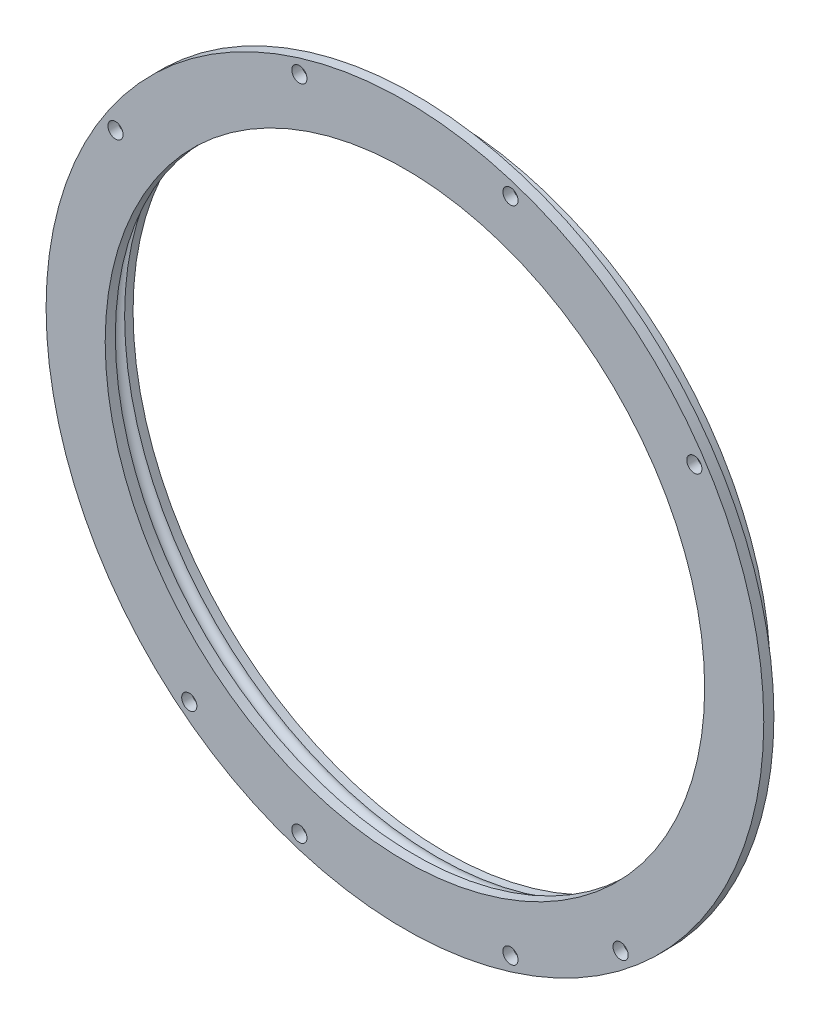
SolidWorks part; units mm, degrees
ref_plane "前视基准面" through (0, 0, 0) normal (0, 0, 1) x (1, 0, 0)
ref_plane "上视基准面" through (0, 0, 0) normal (0, 1, 0) x (1, 0, 0)
ref_plane "右视基准面" through (0, 0, 0) normal (1, 0, 0) x (0, 0, -1)
sketch "草图1" plane through (0, 0, 0) normal (0, 0, 1) x (1, 0, 0)
  circle A0 centre (0, 0) radius 425
  circle A1 centre (0, 0) radius 355
  circle A2 centre (0, 0) radius 409 construction
  dimension "D1" = 850
  dimension "D2" = 710
  dimension "D3" = 818
extrude "凸台-拉伸2" add sketch "草图1" along normal blind 12
sketch "草图3" plane through (0, 0, 0) normal (0, 0, -1) x (-1, 0, 0)
  circle A0 centre (0, 0) radius 370
  circle A1 centre (0, 0) radius 355 construction
  circle A2 centre (0, 0) radius 385
  dimension "D1" = 15
  dimension "D2" = 15
extrude "凸台-拉伸3" add sketch "草图3" along normal blind 36
ref_plane "基准面1" through (0, 0, -18) normal (0, 0, 1) x (1, 0, 0)
sketch "草图4" plane through (0, 0, -18) normal (0, 0, 1) x (1, 0, 0)
  circle A0 centre (0, 0) radius 370
  circle A2 centre (0, 0) radius 370 construction
sweep "切除-扫描2" cut path "草图4" circular profile diameter 16 parameters "D3"=16
hole_wizard "M10x1.0 螺纹孔1" positions "草图21" profile "草图23" tap size "M10x1.0" standard "GB"
sketch "草图21" plane through (0, 0, 0) normal (1, 0, 0) x (0, 0, -1)
  line L0 (18, 370) -> (18, -370) construction
  point P0 (18, 0)
sketch "草图23" plane through (0, 0, -18) normal (0, 1, 0) x (0, 0, 1)
  line L0 (0, 0) -> (0, 385)
  line L1 (0, 385) -> (4.5, 385)
  line L2 (4.5, 385) -> (4.5, 0)
  line L5 (4.5, 0) -> (0, 0)
  line L11 (0, -6.35) -> (0, 107.95) construction
  dimension "通孔螺纹孔钻头直径" = 9
  dimension "通孔螺纹孔钻头深度" = 385
cosmetic thread "孔螺蚊线1" parameters "D2"=10
sketch "草图24" plane through (0, 0, 0) normal (0, 0, -1) x (-1, 0, 0)
  circle A0 centre (0, 0) radius 409 construction
  circle A1 centre (-125, -389.4304) radius 9
  circle A2 centre (125, -389.4304) radius 9
  circle A3 centre (-255.409, -319.4483) radius 9
  circle A4 centre (255.409, -319.4483) radius 9
  circle A6 centre (-125, 389.4304) radius 9
  circle A7 centre (125, 389.4304) radius 9
  circle A8 centre (342.7684, 223.1386) radius 9
  circle A9 centre (-342.7684, 223.1386) radius 9
  dimension "D1" = 18
  dimension "D10" = 818
  dimension "D2" = 250
  dimension "D3" = 125
  dimension "D4" = 148
  dimension "D5" = 148
  dimension "D6" = 250
  dimension "D7" = 125
  dimension "D8" = 274
  dimension "D9" = 274
extrude "切除-拉伸1" cut sketch "草图24" against normal blind 15
